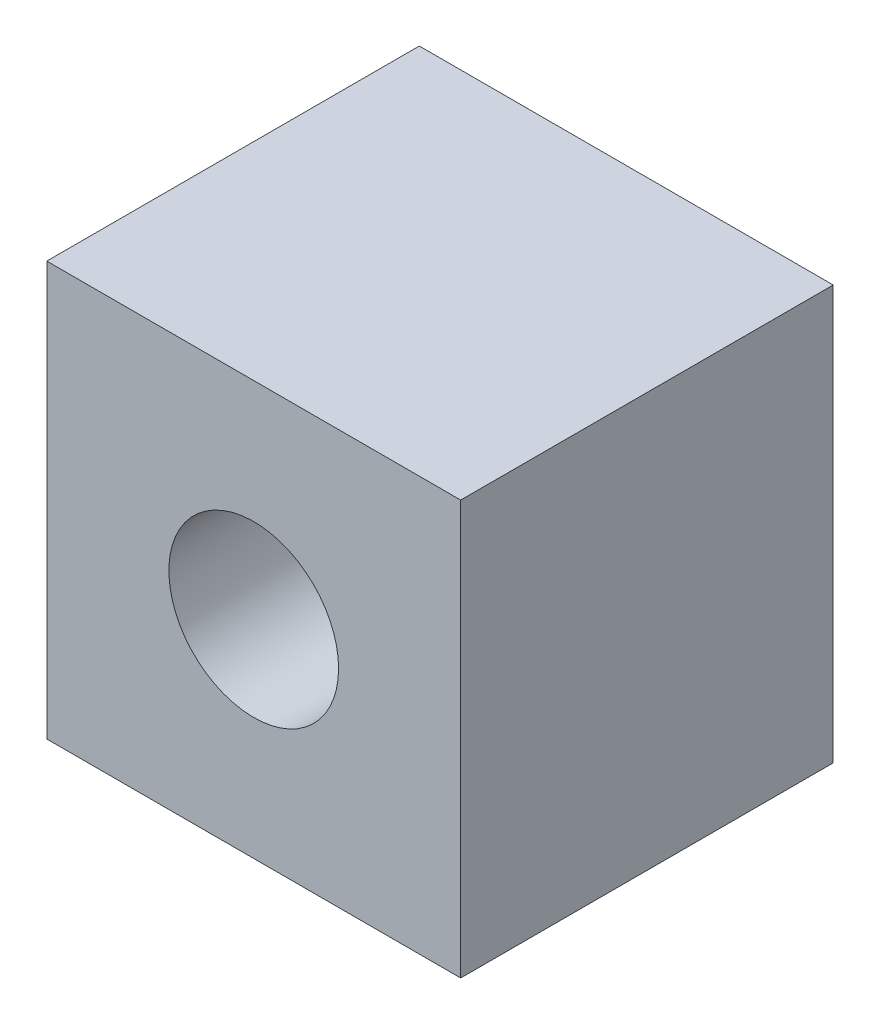
from build123d import *

# Parameters (mm, degrees)
SKETCH_1_W          = 40
SKETCH_1_H          = 40
EXTRUDE_1_DEPTH     = 18
SKETCH_2_R          = 8.2
CUT_EXTRUDE_1_DEPTH = 30


with BuildPart() as part:
    # 草图1 → 凸台-拉伸1 (new, symmetric)
    with BuildSketch(Plane.XY):
        Rectangle(SKETCH_1_W, SKETCH_1_H)
    extrude(amount=EXTRUDE_1_DEPTH, both=True)

    # 草图2 → 切除-拉伸1 (cut, symmetric)
    with BuildSketch(Plane.XY):
        Circle(SKETCH_2_R)
    extrude(amount=CUT_EXTRUDE_1_DEPTH, both=True, mode=Mode.SUBTRACT)


solid = part.part
